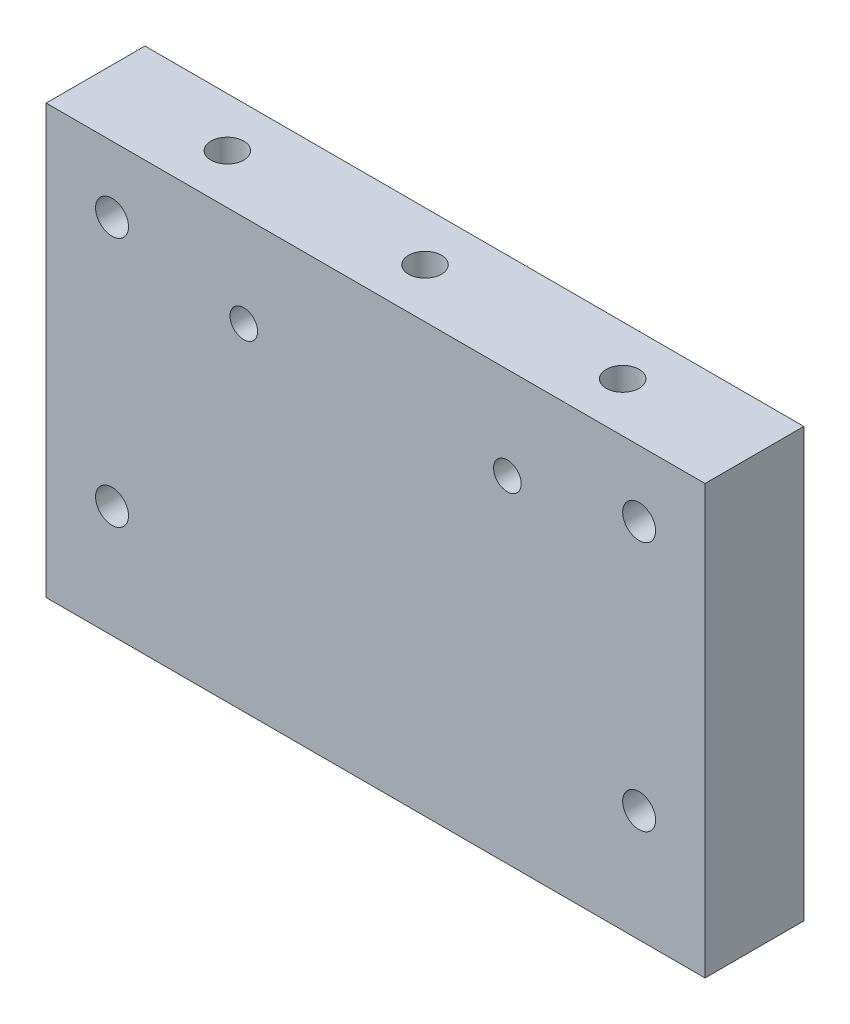
SolidWorks part; units mm, degrees
ref_plane "前视基准面" through (0, 0, 0) normal (0, 0, 1) x (1, 0, 0)
ref_plane "上视基准面" through (0, 0, 0) normal (0, 1, 0) x (1, 0, 0)
ref_plane "右视基准面" through (0, 0, 0) normal (1, 0, 0) x (0, 0, -1)
sketch "草图1" plane through (0, 0, 0) normal (0, 0, 1) x (1, 0, 0)
  line L1 (0, 0) -> (100, 0)
  line L2 (0, 0) -> (0, 65)
  line L3 (0, 65) -> (100, 65)
  line L4 (100, 0) -> (100, 65)
  dimension "D1" = 100
  dimension "D2" = 65
extrude "凸台-拉伸1" add sketch "草图1" along normal blind 15
hole_wizard "M6 螺纹孔1" positions "草图3" profile "草图4" tap size "M6" standard "GB"
sketch "草图3" plane through (0, 65, 0) normal (0, 1, 0) x (1, 0, 0)
  line L0 (0, -7.5) -> (105.8243, -7.5) construction
  line L1 (0, -15) -> (0, 0) construction
  line L3 (50, -15) -> (50, 7.2539) construction
  line L4 (100, -15) -> (0, -15) construction
  point P0 (20, -7.5)
  point P2 (80, -7.5)
  point P4 (50, -7.5)
  dimension "D1" = 60
sketch "草图4" plane through (20, 65, 7.5) normal (1, 0, 0) x (0, 0, 1)
  line L0 (0, 0) -> (0, 16.5022)
  line L1 (0, 16.5022) -> (2.5, 15)
  line L2 (2.5, 15) -> (2.5, 0)
  line L5 (2.5, 0) -> (0, 0)
  line L10 (0, 16.5022) -> (-2.5, 15) construction
  line L11 (0, -6.35) -> (0, 107.95) construction
  dimension "螺纹孔钻头直径" = 5
  dimension "螺纹孔钻头深度" = 15
  dimension "导头角度" = 118
cosmetic thread "孔螺蚊线1" parameters "D1"=12, "D2"=6
cosmetic thread "孔螺蚊线2" parameters "D1"=12, "D2"=6
cosmetic thread "孔螺蚊线3" parameters "D1"=12, "D2"=6
hole_wizard "M6 螺纹孔2" positions "草图5" profile "草图6" tap size "M6" standard "GB"
sketch "草图5" plane through (0, 0, 0) normal (0, -1, 0) x (-1, 0, 0)
  point P0 (-80, -7.5)
  point P3 (-50, -7.5)
  point P6 (-20, -7.5)
sketch "草图6" plane through (80, 0, 7.5) normal (1, 0, 0) x (0, 0, -1)
  line L0 (0, 0) -> (0, 16.5022)
  line L1 (0, 16.5022) -> (2.5, 15)
  line L2 (2.5, 15) -> (2.5, 0)
  line L5 (2.5, 0) -> (0, 0)
  line L10 (0, 16.5022) -> (-2.5, 15) construction
  line L11 (0, -6.35) -> (0, 107.95) construction
  dimension "螺纹孔钻头直径" = 5
  dimension "螺纹孔钻头深度" = 15
  dimension "导头角度" = 118
cosmetic thread "孔螺蚊线4"
cosmetic thread "孔螺蚊线5"
cosmetic thread "孔螺蚊线6"
hole_wizard "M5 螺纹孔1" positions "草图7" profile "草图8" tap size "M5" standard "GB" end condition through all
sketch "草图7" plane through (0, 0, 0) normal (0, 0, -1) x (-1, 0, 0)
  line L0 (-50, 0) -> (-50, 52.6244) construction
  line L1 (0, 0) -> (-100, 0) construction
  point P0 (-70, 51)
  point P2 (-30, 51)
  dimension "D1" = 40
  dimension "D2" = 51
sketch "草图8" plane through (70, 51, 0) normal (1, 0, 0) x (0, 1, 0)
  line L0 (0, 0) -> (0, 15)
  line L1 (0, 15) -> (2.1, 15)
  line L2 (2.1, 15) -> (2.1, 0.425)
  line L3 (2.1, 0.425) -> (2.525, 0)
  line L5 (2.525, 0) -> (0, 0)
  line L6 (-2.1, 0.425) -> (-2.525, 0) construction
  line L11 (0, -6.35) -> (0, 107.95) construction
  dimension "通孔螺纹孔钻头直径" = 4.2
  dimension "通孔螺纹孔钻头深度" = 15
  dimension "近端锥形沉头孔直径" = 5.05
  dimension "近端锥形沉头孔角度" = 90
cosmetic thread "孔螺蚊线7"
cosmetic thread "孔螺蚊线8"
hole_wizard "M6 螺纹孔3" positions "草图9" profile "草图10" tap size "M6" standard "GB" end condition through all
sketch "草图9" plane through (0, 0, 0) normal (0, 0, -1) x (-1, 0, 0)
  line L0 (-50, 0) -> (-50, 70.0474) construction
  line L1 (0, 0) -> (-100, 0) construction
  line L3 (-100, 65) -> (0, 65) construction
  point P0 (-90, 55)
  point P2 (-10, 55)
  point P4 (-90, 17)
  point P6 (-10, 17)
  dimension "D1" = 80
  dimension "D2" = 38
  dimension "D3" = 10
sketch "草图10" plane through (90, 55, 0) normal (1, 0, 0) x (0, 1, 0)
  line L0 (0, 0) -> (0, 15)
  line L1 (0, 15) -> (2.5, 15)
  line L2 (2.5, 15) -> (2.5, 0)
  line L5 (2.5, 0) -> (0, 0)
  line L11 (0, -6.35) -> (0, 107.95) construction
  dimension "通孔螺纹孔钻头直径" = 5
  dimension "通孔螺纹孔钻头深度" = 15
cosmetic thread "孔螺蚊线9"
cosmetic thread "孔螺蚊线10"
cosmetic thread "孔螺蚊线11"
cosmetic thread "孔螺蚊线12"
